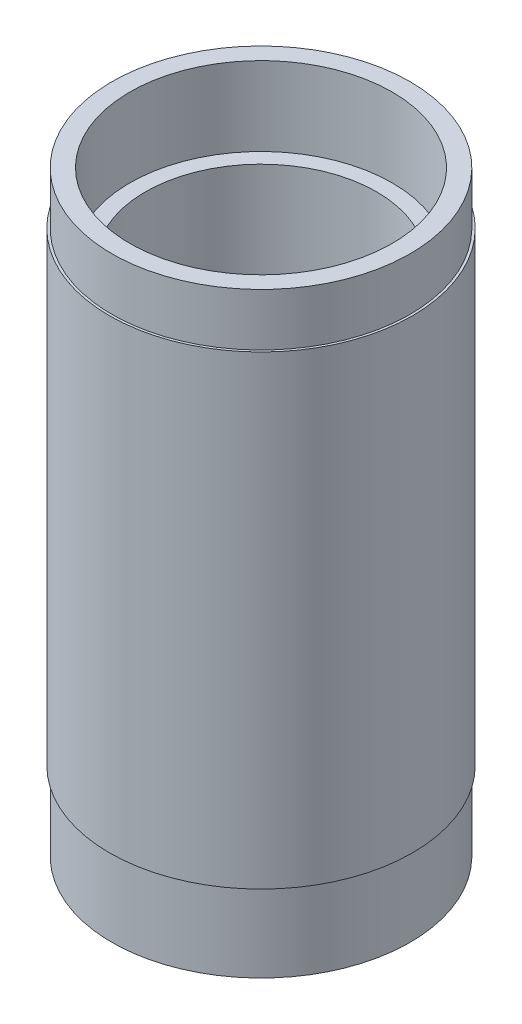
SolidWorks part; units mm, degrees
material "Q235B"
ref_plane "Front Plane" through (0, 0, 0) normal (0, 0, 1) x (1, 0, 0)
ref_plane "Top Plane" through (0, 0, 0) normal (0, 1, 0) x (1, 0, 0)
ref_plane "Right Plane" through (0, 0, 0) normal (1, 0, 0) x (0, 0, -1)
sketch "Sketch1" plane through (0, 0, 0) normal (0, 0, 1) x (1, 0, 0)
  line L0 (55, 0) -> (55, 33)
  line L1 (55, 33) -> (48.5, 33)
  line L2 (48.5, 33) -> (48.5, 217)
  line L3 (48.5, 217) -> (55, 217)
  line L4 (55, 217) -> (55, 250)
  line L5 (55, 250) -> (62.5, 250)
  line L6 (62.5, 250) -> (62.5, 228)
  line L7 (62.5, 228) -> (63.5, 228)
  line L8 (63.5, 228) -> (63.5, 33)
  line L9 (63.5, 33) -> (62.5, 33)
  line L10 (62.5, 33) -> (62.5, 0)
  line L11 (62.5, 0) -> (55, 0)
  line L12 (0, 0) -> (0, 198.9409) construction
  dimension "D1" = 110
  dimension "D2" = 33
  dimension "D3" = 33
  dimension "D4" = 97
  dimension "D5" = 110
  dimension "D6" = 125
  dimension "D7" = 127
  dimension "D8" = 22
  dimension "D9" = 33
  dimension "D10" = 250
revolve "Revolve1" add sketch "Sketch1" angle 360 about L12
